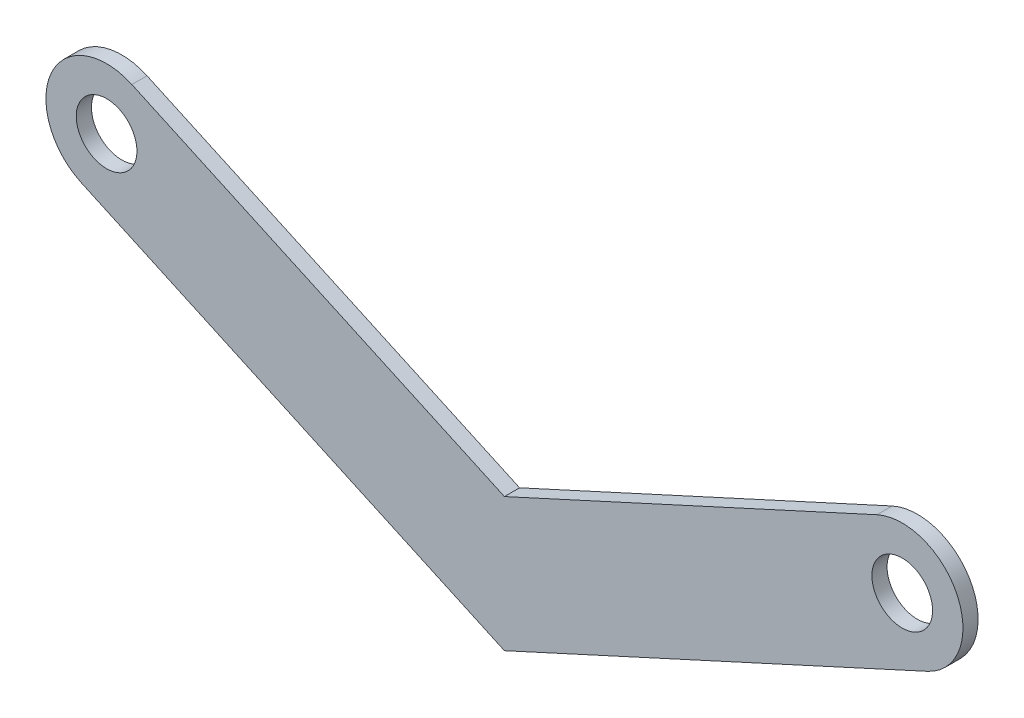
from build123d import *

# Parameters (mm, degrees)
SKETCH1_R           = 5
BOSS_EXTRUDE1_DEPTH = 2.5


with BuildPart() as part:
    # Sketch1 → Boss-Extrude1 (new body)
    with BuildSketch(Plane.XY):
        with BuildLine():
            Line((0, 21.995608), (61.387985551, 50.094742382))
            ThreePointArc((61.387985551, 50.094742382), (74.642724329, 45.164032502), (69.712014449, 31.909293724))
            Line((69.712014449, 31.909293724), (0, 0))
            Line((0, 0), (-69.712014449, 31.909293724))
            ThreePointArc((-69.712014449, 31.909293724), (-74.642724329, 45.164032502), (-61.387985551, 50.094742382))
            Line((-61.387985551, 50.094742382), (0, 21.995608))
        make_face()
        with Locations((-65.55, 41.002018053)):
            Circle(SKETCH1_R, mode=Mode.SUBTRACT)
        with Locations((65.55, 41.002018053)):
            Circle(SKETCH1_R, mode=Mode.SUBTRACT)
    extrude(amount=BOSS_EXTRUDE1_DEPTH)


solid = part.part
